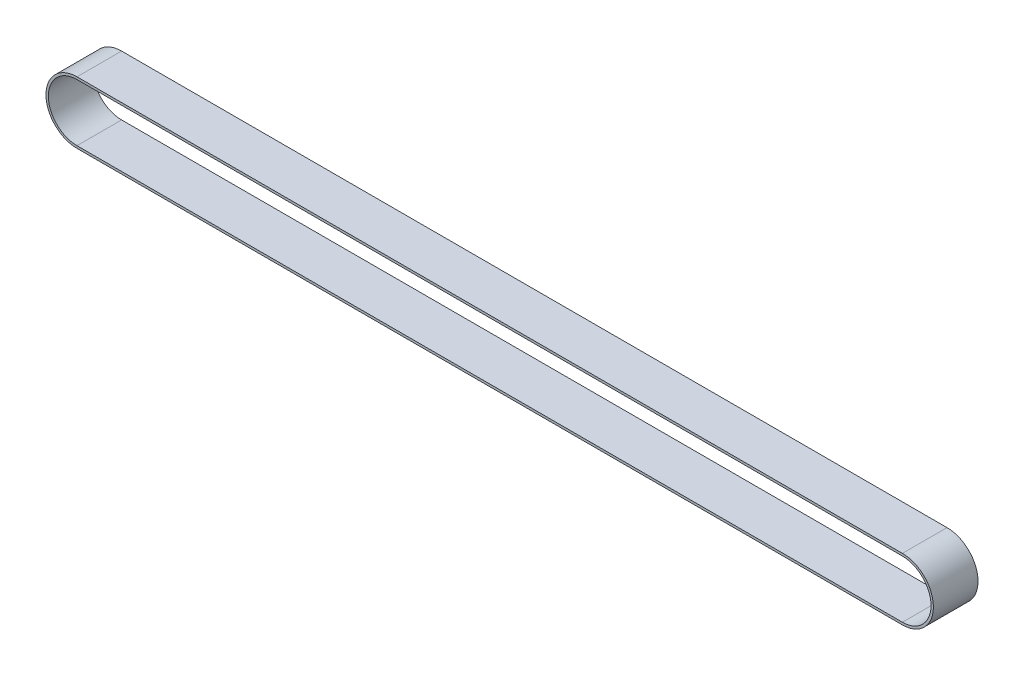
from build123d import *

# Parameters (mm, degrees)
EXTRUDE_1_DEPTH = 6


with BuildPart() as part:
    # 草图1 → 凸台-拉伸1 (new, symmetric)
    with BuildSketch(Plane.XY):
        with BuildLine():
            Line((0, 8.335), (222, 8.335))
            ThreePointArc((222, 8.335), (230.335, 0), (222, -8.335))
            Line((222, -8.335), (0, -8.335))
            ThreePointArc((0, -8.335), (-8.335, 0), (0, 8.335))
        make_face()
        with BuildLine():
            Line((0, 7.705), (222, 7.705))
            ThreePointArc((222, 7.705), (229.705, 0), (222, -7.705))
            Line((222, -7.705), (0, -7.705))
            ThreePointArc((0, -7.705), (-7.705, 0), (0, 7.705))
        make_face(mode=Mode.SUBTRACT)
    extrude(amount=EXTRUDE_1_DEPTH, both=True)


solid = part.part
